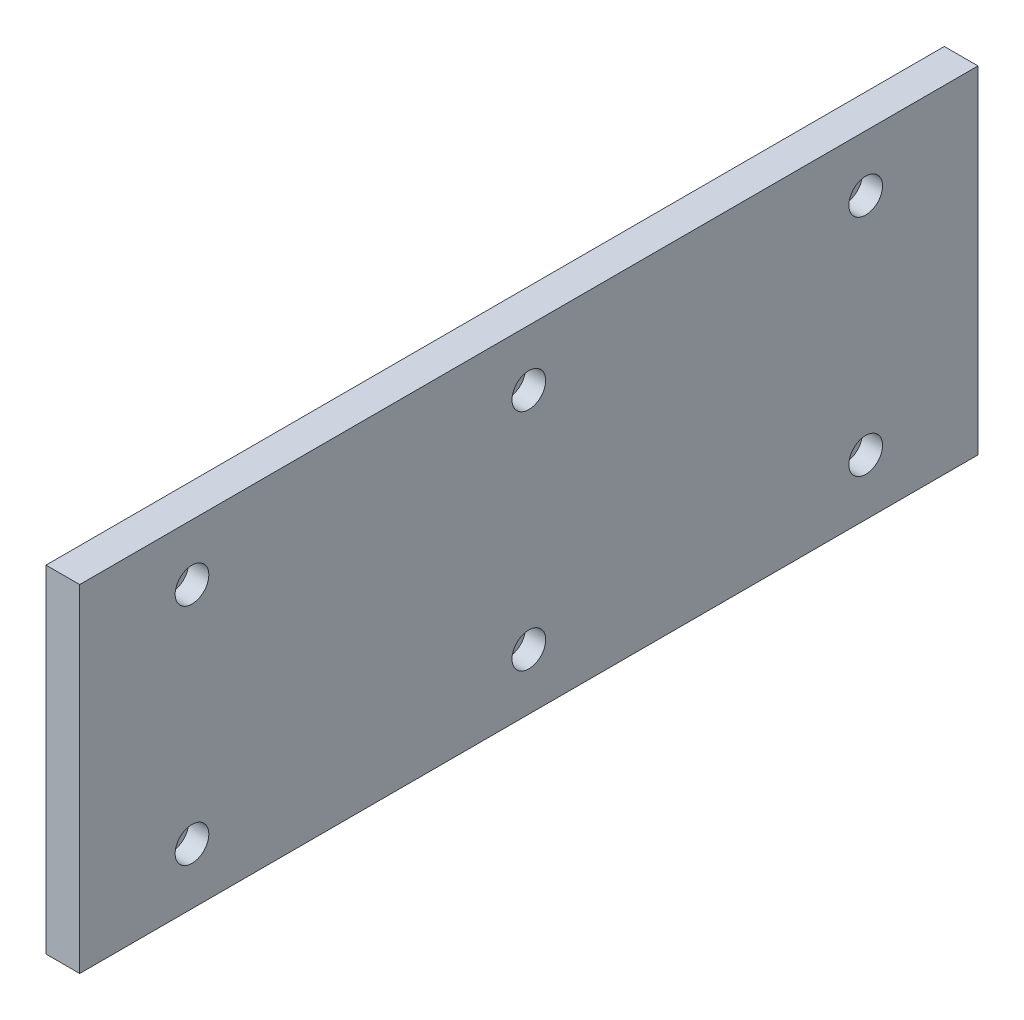
SolidWorks part; units mm, degrees
ref_plane "前视基准面" through (0, 0, 0) normal (0, 0, 1) x (1, 0, 0)
ref_plane "上视基准面" through (0, 0, 0) normal (0, 1, 0) x (1, 0, 0)
ref_plane "右视基准面" through (0, 0, 0) normal (1, 0, 0) x (0, 0, -1)
sketch "草图1" plane through (0, 0, 0) normal (1, 0, 0) x (0, 0, -1)
  line L1 (-200, 75) -> (200, 75)
  line L2 (-200, 75) -> (-200, -75)
  line L3 (-200, -75) -> (200, -75)
  line L4 (200, 75) -> (200, -75)
  line L5 (-200, 75) -> (200, -75) construction
  line L6 (-200, -75) -> (200, 75) construction
  point P0 (0, 0)
  dimension "D1" = 400
  dimension "D2" = 150
extrude "凸台-拉伸1" add sketch "草图1" along normal blind 15
hole_wizard "打孔尺寸(%根据)内六角圆柱头螺钉的类型1" positions "草图2" profile "草图3" counterbore size "M8" standard "GB" end condition through all
sketch "草图2" plane through (15, 0, 0) normal (1, 0, 0) x (0, 0, -1)
  line L0 (0, 138.1478) -> (0, 0) construction
  line L1 (0, 0) -> (226.2328, 0) construction
  point P0 (-150, 50)
  point P2 (0, 50)
  point P4 (150, 50)
  point P6 (-150, -50)
  point P8 (0, -50)
  point P10 (150, -50)
  dimension "D1" = 300
  dimension "D2" = 100
sketch "草图3" plane through (15, 50, 150) normal (0, 1, 0) x (0, 0, -1)
  line L0 (0, 0) -> (0, 15)
  line L1 (0, 15) -> (4.5, 15)
  line L3 (4.5, 15) -> (4.5, 9)
  line L4 (4.5, 9) -> (7.5, 9)
  line L5 (7.5, 9) -> (7.5, 0)
  line L7 (7.5, 0) -> (0, 0)
  line L11 (0, -6.35) -> (0, 107.95) construction
  dimension "通孔孔直径" = 9
  dimension "通孔孔深度" = 15
  dimension "柱形沉头孔直径" = 15
  dimension "柱形沉头孔深度" = 9
